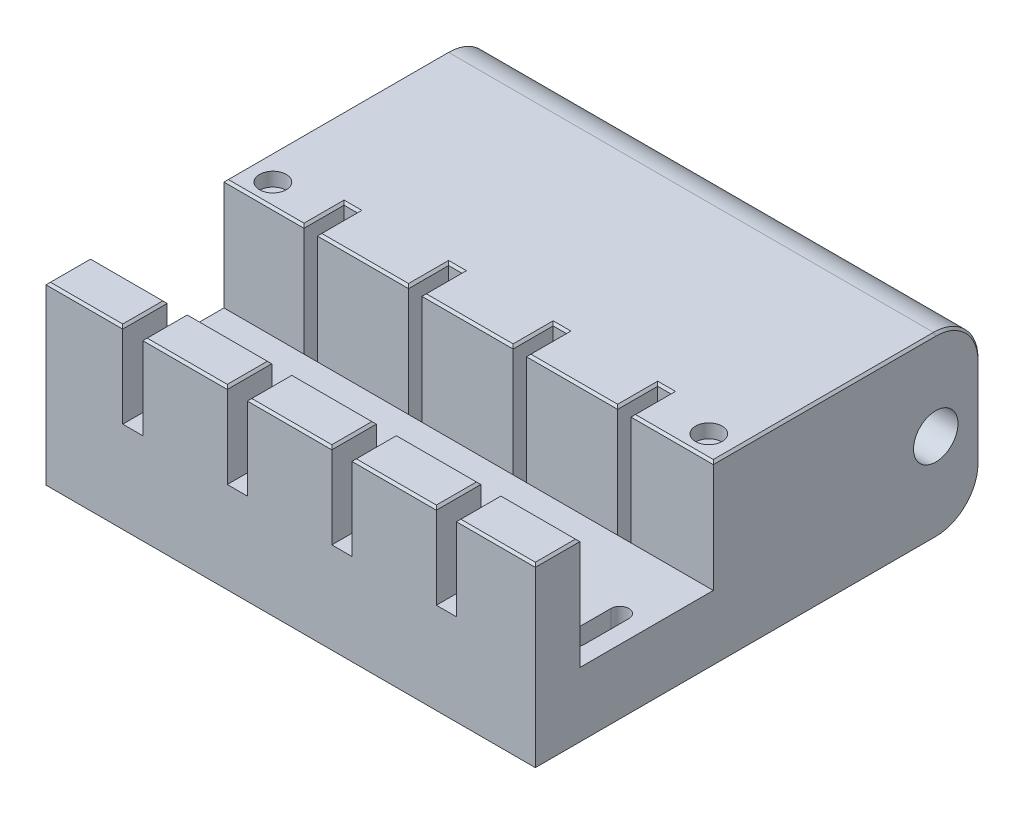
from build123d import *

# Parameters (mm, degrees)
SKETCH7_W                = 110
SKETCH7_H                = 100
BOSS_EXTRUDE2_DEPTH      = 40
SKETCH8_W                = 3
SKETCH8_H                = 9
CUT_EXTRUDE1_DEPTH       = 85.409715081
SKETCH11_W               = 4.5
SKETCH11_H               = 17
CUT_EXTRUDE4_DEPTH       = 19
SKETCH9_W                = 30
SKETCH9_H                = 25
CUT_EXTRUDE5_DEPTH       = 128.279220614
SKETCH12_R               = 5
CUT_EXTRUDE6_DEPTH       = 128.279220614
F_4_0_4_DIAMETER_HOLE1_D = 4
CUT_EXTRUDE8_DEPTH       = 85.409715081
CUT_EXTRUDE9_DEPTH       = 5
FILLET1_R                = 10
CHAMFER1_SIZE            = 0.5
CHAMFER2_SIZE            = 0.5
CHAMFER3_SIZE            = 0.5
SKETCH20_R               = 3
CUT_EXTRUDE10_DEPTH      = 3.1


with BuildPart() as part:
    # Sketch7 → Boss-Extrude2 (new body)
    with BuildSketch(Plane(origin=(0, 0, 0), x_dir=(1, 0, 0), z_dir=(0, 1, 0))):
        Rectangle(SKETCH7_W, SKETCH7_H)
    extrude(amount=BOSS_EXTRUDE2_DEPTH)

    # Sketch8 → Cut-Extrude1 (cut, through all)
    with BuildSketch(Plane(origin=(0, 40, 0), x_dir=(1, 0, 0), z_dir=(0, 1, 0))):
        with Locations((-35.5, -5.5)):
            Rectangle(SKETCH8_W, SKETCH8_H)
        with Locations((-12, -5.5)):
            Rectangle(SKETCH8_W, SKETCH8_H)
        with Locations((11.5, -5.5)):
            Rectangle(SKETCH8_W, SKETCH8_H)
        with Locations((35, -5.5)):
            Rectangle(SKETCH8_W, SKETCH8_H)
    extrude(amount=-CUT_EXTRUDE1_DEPTH, mode=Mode.SUBTRACT)

    # Sketch11 → Cut-Extrude4 (cut)
    with BuildSketch(Plane(origin=(0, 40, 0), x_dir=(1, 0, 0), z_dir=(0, 1, 0))):
        with Locations((-35.5, -43.5)):
            Rectangle(SKETCH11_W, SKETCH11_H)
        with Locations((-12, -43.5)):
            Rectangle(SKETCH11_W, SKETCH11_H)
        with Locations((11.5, -43.5)):
            Rectangle(SKETCH11_W, SKETCH11_H)
        with Locations((35, -43.5)):
            Rectangle(SKETCH11_W, SKETCH11_H)
    extrude(amount=-CUT_EXTRUDE4_DEPTH, mode=Mode.SUBTRACT)

    # Sketch9 → Cut-Extrude5 (cut, through all)
    with BuildSketch(Plane(origin=(55, 0, 0), x_dir=(0, 0, -1), z_dir=(1, 0, 0))):
        with Locations((-25, 27.5)):
            Rectangle(SKETCH9_W, SKETCH9_H)
    extrude(amount=-CUT_EXTRUDE5_DEPTH, mode=Mode.SUBTRACT)

    # Sketch12 → Cut-Extrude6 (cut, through all)
    with BuildSketch(Plane(origin=(55, 0, 0), x_dir=(0, 0, -1), z_dir=(1, 0, 0))):
        with Locations((40, 20)):
            Circle(SKETCH12_R)
    extrude(amount=-CUT_EXTRUDE6_DEPTH, mode=Mode.SUBTRACT)

    # Ø4.0 (4) Diameter Hole1 (through all)
    with Locations(Plane(origin=(0, 21, 0), x_dir=(1, 0, 0), z_dir=(0, 1, 0))):
        with Locations((-49, -35), (49, -35)):
            Hole(F_4_0_4_DIAMETER_HOLE1_D / 2)

    # Sketch18 → Cut-Extrude8 (cut, through all)
    with BuildSketch(Plane.XZ):
        with BuildLine():
            Line((-47, 35), (-47, 25))
            ThreePointArc((-47, 25), (-49, 23), (-51, 25))
            Line((-51, 25), (-51, 35))
            ThreePointArc((-51, 35), (-49, 37), (-47, 35))
        make_face()
        with BuildLine():
            Line((47, 35), (47, 25))
            ThreePointArc((47, 25), (49, 23), (51, 25))
            Line((51, 25), (51, 35))
            ThreePointArc((51, 35), (49, 37), (47, 35))
        make_face()
    extrude(amount=-CUT_EXTRUDE8_DEPTH, mode=Mode.SUBTRACT)

    # Sketch19 → Cut-Extrude9 (cut)
    with BuildSketch(Plane.XZ):
        with BuildLine():
            Line((-53, 35), (-53, 25))
            ThreePointArc((-53, 25), (-49, 21), (-45, 25))
            Line((-45, 25), (-45, 35))
            ThreePointArc((-45, 35), (-49, 39), (-53, 35))
        make_face()
        with BuildLine():
            Line((45, 35), (45, 25))
            ThreePointArc((45, 25), (49, 21), (53, 25))
            Line((53, 25), (53, 35))
            ThreePointArc((53, 35), (49, 39), (45, 35))
        make_face()
    extrude(amount=-CUT_EXTRUDE9_DEPTH, mode=Mode.SUBTRACT)

    # Fillet1
    fillet1_edges = [part.edges().sort_by_distance(p)[0] for p in [
        (0, 0, -50),
        (0, 40, -50),
    ]]
    fillet(fillet1_edges, radius=FILLET1_R)

    # Chamfer1
    chamfer1_edges = [part.edges().sort_by_distance(p)[0] for p in [
        (0, 0, 50),
    ]]
    chamfer(chamfer1_edges, length=CHAMFER1_SIZE)

    # Chamfer2
    chamfer2_edges = [part.edges().sort_by_distance(p)[0] for p in [
        (-55, 0, 4.75),
        (55, 0, 4.75),
        (-55, 2.928932188, -47.071067812),
        (55, 2.928932188, -47.071067812),
        (-55, 20, -50),
        (55, 20, -50),
        (-55, 37.071067812, -47.071067812),
        (55, 37.071067812, -47.071067812),
        (-55, 40, -15),
        (-46, 40, 10),
        (-37, 40, 5.5),
        (-35.5, 40, 1),
        (-34, 40, 5.5),
        (-23.75, 40, 10),
        (-13.5, 40, 5.5),
        (-12, 40, 1),
        (-10.5, 40, 5.5),
        (-0.25, 40, 10),
        (10, 40, 5.5),
        (11.5, 40, 1),
        (13, 40, 5.5),
        (23.25, 40, 10),
        (33.5, 40, 5.5),
        (35, 40, 1),
        (36.5, 40, 5.5),
        (45.75, 40, 10),
        (55, 40, -15),
    ]]
    chamfer(chamfer2_edges, length=CHAMFER2_SIZE)

    # Chamfer3
    chamfer3_edges = [part.edges().sort_by_distance(p)[0] for p in [
        (-37.75, 40, 45),
        (-14.25, 40, 45),
        (9.25, 40, 45),
        (32.75, 40, 45),
        (-55, 40, 45),
        (-46.375, 40, 50),
        (46.125, 40, 40),
        (-46.375, 40, 40),
        (-23.75, 40, 40),
        (-0.25, 40, 40),
        (23.25, 40, 40),
        (55, 40, 45),
        (-23.75, 40, 50),
        (-0.25, 40, 50),
        (23.25, 40, 50),
        (46.125, 40, 50),
        (37.25, 40, 45),
        (13.75, 40, 45),
        (-9.75, 40, 45),
        (-33.25, 40, 45),
    ]]
    chamfer(chamfer3_edges, length=CHAMFER3_SIZE)

    # Sketch20 → Cut-Extrude10 (cut)
    with BuildSketch(Plane(origin=(0, 40, 0), x_dir=(1, 0, 0), z_dir=(0, 1, 0))):
        with Locations(Location((-49, -5, 0), (0, 0, 270))):
            Circle(SKETCH20_R)
        with Locations(Location((49, -5, 0), (0, 0, 270))):
            Circle(SKETCH20_R)
    extrude(amount=-CUT_EXTRUDE10_DEPTH, mode=Mode.SUBTRACT)


solid = part.part
